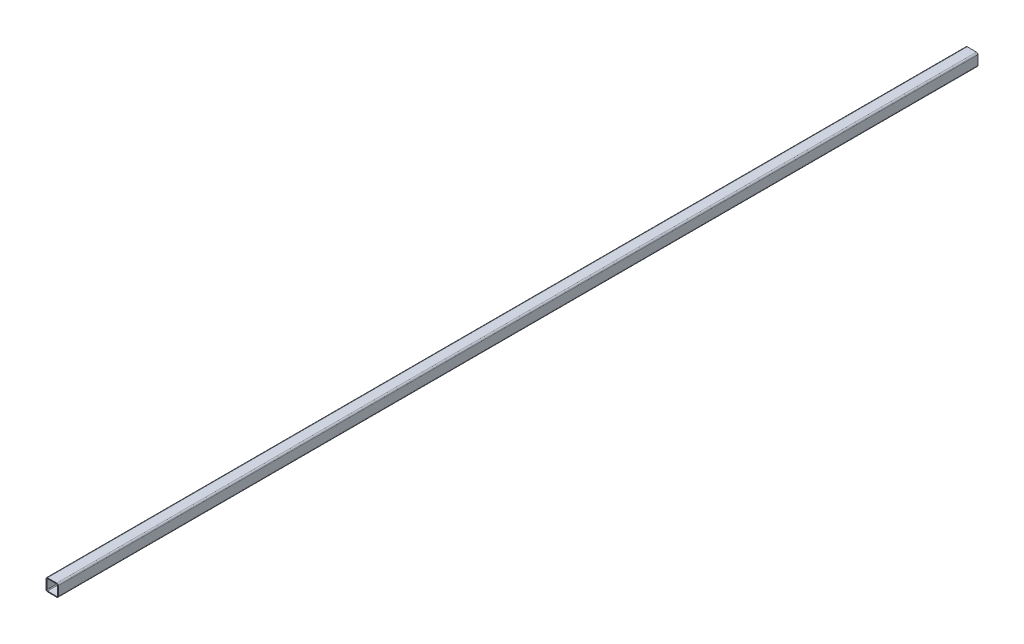
SolidWorks part; units mm, degrees
ref_plane "Front Plane" through (0, 0, 0) normal (0, 0, 1) x (1, 0, 0)
ref_plane "Top Plane" through (0, 0, 0) normal (0, 1, 0) x (1, 0, 0)
ref_plane "Right Plane" through (0, 0, 0) normal (1, 0, 0) x (0, 0, -1)
sketch "Sketch 1" plane through (0, 0, 0) normal (0, 0, 1) x (1, 0, 0)
  line L0 (0, 96.8978) -> (0, -107.4818) construction
  line L1 (-129.1971, 0) -> (137.9562, 0) construction
  line L2 (0, 32) -> (-24, 32)
  line L3 (-32, 24) -> (-32, 0)
  line L4 (0, 28) -> (-24, 28)
  line L5 (-28, 24) -> (-28, 0)
  line L6 (-28, -24) -> (-28, 0)
  line L7 (24, -28) -> (-24, -28)
  line L8 (-32, -24) -> (-32, 0)
  line L9 (24, -32) -> (-24, -32)
  line L10 (32, -24) -> (32, 0)
  line L11 (28, -24) -> (28, 0)
  line L12 (28, 24) -> (28, 0)
  line L13 (0, 28) -> (24, 28)
  line L14 (32, 24) -> (32, 0)
  line L15 (0, 32) -> (24, 32)
  arc A0 (-24, 32) -> (-32, 24) centre (-24, 24) ccw
  arc A1 (-24, 28) -> (-28, 24) centre (-24, 24) ccw
  arc A2 (-24, -28) -> (-28, -24) centre (-24, -24) cw
  arc A3 (-24, -32) -> (-32, -24) centre (-24, -24) cw
  arc A4 (24, -32) -> (32, -24) centre (24, -24) ccw
  arc A5 (24, -28) -> (28, -24) centre (24, -24) ccw
  arc A6 (24, 28) -> (28, 24) centre (24, 24) cw
  arc A7 (24, 32) -> (32, 24) centre (24, 24) cw
  point P34 (0, -32)
  point P35 (0, -28)
  dimension "D3" = 8
  dimension "D1" = 64
  dimension "D2" = 64
  dimension "D4" = 4
extrude "Boss-Extrude 1" add sketch "Sketch 1" along normal mid plane 4800
